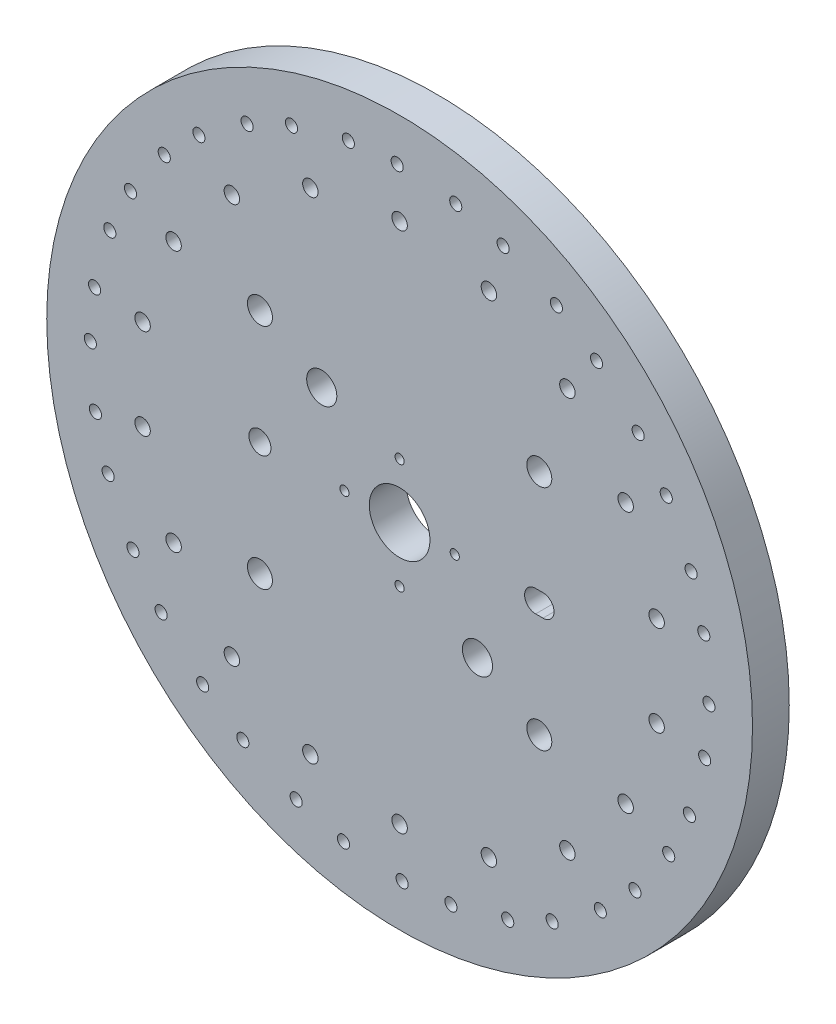
SolidWorks part; units mm, degrees
material "AISI 304"
ref_plane "Front Plane" through (0, 0, 0) normal (0, 0, 1) x (1, 0, 0)
ref_plane "Top Plane" through (0, 0, 0) normal (0, 1, 0) x (1, 0, 0)
ref_plane "Right Plane" through (0, 0, 0) normal (1, 0, 0) x (0, 0, -1)
sketch "Sketch1" plane through (0, 0, 0) normal (0, 0, 1) x (1, 0, 0)
  circle A0 centre (0, 0) radius 102.5
  dimension "D1" = 205
extrude "Boss-Extrude1" add sketch "Sketch1" along normal blind 10
sketch "Sketch2" plane through (0, 0, 0) normal (0, 0, -1) x (-1, 0, 0)
  circle A0 centre (0, 0) radius 8.25
  dimension "D1" = 16.5
extrude "Cut-Extrude1" cut sketch "Sketch2" against normal through all
sketch "Sketch4" plane through (0, 0, 0) normal (0, 0, -1) x (-1, 0, 0)
  line L0 (0, 0) -> (0, -50000) construction
  line L1 (0, 0) -> (-12940.9523, -48296.2913) construction
  circle A0 centre (0, 0) radius 84.145 construction
  circle A1 centre (-29.4071, -78.8391) radius 1
  circle A2 centre (-13.9523, -82.9802) radius 1
  dimension "D1" = 168.29
  dimension "D2" = 16
  dimension "D3" = 2
  dimension "D4" = 15
extrude "Cut-Extrude3" cut sketch "Sketch4" against normal blind 20
pattern_circular "CirPattern2" count 18 over 360 about axis through (0, 0, 0) along (0, 0, 1) of "Cut-Extrude3"
sketch "Sketch5" plane through (0, 0, 0) normal (0, 0, -1) x (-1, 0, 0)
  line L0 (0, 0) -> (0, 50000) construction
  circle A0 centre (0, 0) radius 71 construction
  circle A1 centre (0, -71) radius 2.1
  dimension "D1" = 142
  dimension "D2" = 4.2
extrude "Cut-Extrude4" cut sketch "Sketch5" against normal through all
pattern_circular "CirPattern3" count 18 over 360 about axis through (0, 0, 0) along (0, 0, 1) of "Cut-Extrude4"
sketch "Sketch7" plane through (0, 0, 0) normal (0, 0, -1) x (-1, 0, 0)
  circle A0 centre (0, 0) radius 96
  circle A1 centre (0, 0) radius 102.5
  dimension "D1" = 192
  dimension "D2" = 205
extrude "Cut-Extrude5" cut sketch "Sketch7" against normal blind 34
hole_wizard "M4 Tapped Hole1" positions "3DSketch3" profile "Sketch20" tap size "M4" standard "Gb" end condition through all
sketch3d "3DSketch3"
  line L0 (-15.2701, -82.7478, 10) -> (-15.2701, -82.7478, 0) construction
  line L1 (-28.1497, -79.2968, 10) -> (-28.1497, -79.2968, 0) construction
  line L2 (-42.6506, -72.5349, 10) -> (-42.6506, -72.5349, 0) construction
  line L3 (-53.5731, -64.8868, 10) -> (-53.5731, -64.8868, 0) construction
  line L4 (-64.8868, -53.5731, 10) -> (-64.8868, -53.5731, 0) construction
  line L5 (-72.5349, -42.6506, 10) -> (-72.5349, -42.6506, 0) construction
  line L6 (-79.2968, -28.1497, 10) -> (-79.2968, -28.1497, 0) construction
  line L7 (-82.7478, -15.2701, 10) -> (-82.7478, -15.2701, 0) construction
  line L8 (-84.1423, 0.6691, 10) -> (-84.1423, 0.6691, 0) construction
  line L9 (-82.9802, 13.9523, 10) -> (-82.9802, 13.9523, 0) construction
  line L10 (-78.8391, 29.4071, 10) -> (-78.8391, 29.4071, 0) construction
  line L11 (-73.2039, 41.4917, 10) -> (-73.2039, 41.4917, 0) construction
  line L12 (-64.0267, 54.5982, 10) -> (-64.0267, 54.5982, 0) construction
  line L13 (-54.5982, 64.0267, 10) -> (-54.5982, 64.0267, 0) construction
  line L14 (-41.4917, 73.2039, 10) -> (-41.4917, 73.2039, 0) construction
  line L15 (-29.4071, 78.8391, 10) -> (-29.4071, 78.8391, 0) construction
  line L16 (-13.9523, 82.9802, 10) -> (-13.9523, 82.9802, 0) construction
  line L17 (-0.6691, 84.1423, 10) -> (-0.6691, 84.1423, 0) construction
  line L18 (15.2701, 82.7478, 10) -> (15.2701, 82.7478, 0) construction
  line L19 (28.1497, 79.2968, 10) -> (28.1497, 79.2968, 0) construction
  line L20 (42.6506, 72.5349, 10) -> (42.6506, 72.5349, 0) construction
  line L21 (53.5731, 64.8868, 10) -> (53.5731, 64.8868, 0) construction
  line L22 (64.8868, 53.5731, 10) -> (64.8868, 53.5731, 0) construction
  line L23 (72.5349, 42.6506, 10) -> (72.5349, 42.6506, 0) construction
  line L24 (79.2968, 28.1497, 10) -> (79.2968, 28.1497, 0) construction
  line L25 (82.7478, 15.2701, 10) -> (82.7478, 15.2701, 0) construction
  line L26 (84.1423, -0.6691, 10) -> (84.1423, -0.6691, 0) construction
  line L27 (82.9802, -13.9523, 10) -> (82.9802, -13.9523, 0) construction
  line L28 (78.8391, -29.4071, 10) -> (78.8391, -29.4071, 0) construction
  line L29 (73.2039, -41.4917, 10) -> (73.2039, -41.4917, 0) construction
  line L30 (64.0267, -54.5982, 10) -> (64.0267, -54.5982, 0) construction
  line L31 (54.5982, -64.0267, 10) -> (54.5982, -64.0267, 0) construction
  line L32 (41.4917, -73.2039, 10) -> (41.4917, -73.2039, 0) construction
  line L33 (29.4071, -78.8391, 10) -> (29.4071, -78.8391, 0) construction
  line L34 (13.9523, -82.9802, 10) -> (13.9523, -82.9802, 0) construction
  line L35 (0.6691, -84.1423, 10) -> (0.6691, -84.1423, 0) construction
  point P0 (-15.2701, -82.7478, 10)
  point P5 (-28.1497, -79.2968, 10)
  point P9 (-42.6506, -72.5349, 10)
  point P13 (-53.5731, -64.8868, 10)
  point P17 (-64.8868, -53.5731, 10)
  point P21 (-72.5349, -42.6506, 10)
  point P25 (-79.2968, -28.1497, 10)
  point P29 (-82.7478, -15.2701, 10)
  point P33 (-84.1423, 0.6691, 10)
  point P37 (-82.9802, 13.9523, 10)
  point P41 (-78.8391, 29.4071, 10)
  point P45 (-73.2039, 41.4917, 10)
  point P49 (-64.0267, 54.5982, 10)
  point P53 (-54.5982, 64.0267, 10)
  point P57 (-41.4917, 73.2039, 10)
  point P61 (-29.4071, 78.8391, 10)
  point P65 (-13.9523, 82.9802, 10)
  point P69 (-0.6691, 84.1423, 10)
  point P73 (15.2701, 82.7478, 10)
  point P77 (28.1497, 79.2968, 10)
  point P81 (42.6506, 72.5349, 10)
  point P85 (53.5731, 64.8868, 10)
  point P89 (64.8868, 53.5731, 10)
  point P93 (72.5349, 42.6506, 10)
  point P97 (79.2968, 28.1497, 10)
  point P101 (82.7478, 15.2701, 10)
  point P105 (84.1423, -0.6691, 10)
  point P109 (82.9802, -13.9523, 10)
  point P113 (78.8391, -29.4071, 10)
  point P117 (73.2039, -41.4917, 10)
  point P121 (64.0267, -54.5982, 10)
  point P125 (54.5982, -64.0267, 10)
  point P129 (41.4917, -73.2039, 10)
  point P133 (29.4071, -78.8391, 10)
  point P137 (13.9523, -82.9802, 10)
  point P141 (0.6691, -84.1423, 10)
sketch "Sketch20" plane through (-15.2701, -82.7478, 10) normal (1, 0, 0) x (0, -1, 0)
  line L0 (0, 0) -> (0, 10)
  line L1 (0, 10) -> (1.65, 10)
  line L2 (1.65, 10) -> (1.65, 0)
  line L5 (1.65, 0) -> (0, 0)
  line L11 (0, -6.35) -> (0, 107.95) construction
  dimension "通孔螺纹孔钻头直径" = 3.3
  dimension "通孔螺纹孔钻头深度" = 10
cosmetic thread "Cosmetic thread 17" parameters "D2"=4
cosmetic thread "Cosmetic thread 18" parameters "D2"=4
cosmetic thread "Cosmetic thread 19" parameters "D2"=4
cosmetic thread "Cosmetic thread 20" parameters "D2"=4
cosmetic thread "Cosmetic thread 21" parameters "D2"=4
cosmetic thread "Cosmetic thread 22" parameters "D2"=4
cosmetic thread "Cosmetic thread 23" parameters "D2"=4
cosmetic thread "Cosmetic thread 24" parameters "D2"=4
cosmetic thread "Cosmetic thread 25" parameters "D2"=4
cosmetic thread "Cosmetic thread 26" parameters "D2"=4
cosmetic thread "Cosmetic thread 27" parameters "D2"=4
cosmetic thread "Cosmetic thread 28" parameters "D2"=4
cosmetic thread "Cosmetic thread 29" parameters "D2"=4
cosmetic thread "Cosmetic thread 30" parameters "D2"=4
cosmetic thread "Cosmetic thread 31" parameters "D2"=4
cosmetic thread "Cosmetic thread 32" parameters "D2"=4
cosmetic thread "Cosmetic thread 33" parameters "D2"=4
cosmetic thread "Cosmetic thread 34" parameters "D2"=4
cosmetic thread "Cosmetic thread 35" parameters "D2"=4
cosmetic thread "Cosmetic thread 36" parameters "D2"=4
cosmetic thread "Cosmetic thread 37" parameters "D2"=4
cosmetic thread "Cosmetic thread 38" parameters "D2"=4
cosmetic thread "Cosmetic thread 39" parameters "D2"=4
cosmetic thread "Cosmetic thread 40" parameters "D2"=4
cosmetic thread "Cosmetic thread 41" parameters "D2"=4
cosmetic thread "Cosmetic thread 42" parameters "D2"=4
cosmetic thread "Cosmetic thread 43" parameters "D2"=4
cosmetic thread "Cosmetic thread 44" parameters "D2"=4
cosmetic thread "Cosmetic thread 45" parameters "D2"=4
cosmetic thread "Cosmetic thread 46" parameters "D2"=4
cosmetic thread "Cosmetic thread 47" parameters "D2"=4
cosmetic thread "Cosmetic thread 48" parameters "D2"=4
cosmetic thread "Cosmetic thread 49" parameters "D2"=4
cosmetic thread "Cosmetic thread 50" parameters "D2"=4
cosmetic thread "Cosmetic thread 51" parameters "D2"=4
cosmetic thread "Cosmetic thread 52" parameters "D2"=4
hole_wizard "M8 Tapped Hole2" positions "Sketch40" profile "Sketch39" tap size "M8" standard "Gb" end condition through all
sketch "Sketch40" plane through (0, 0, 10) normal (0, 0, 1) x (1, 0, 0)
  line L0 (0, 0) -> (0, 50000) construction
  line L1 (0, 0) -> (50000, 0) construction
  line L12 (0, 0) -> (35355.3391, 35355.3391) construction
  line L13 (0, 0) -> (38743.251, 31606.3364) construction
  line L14 (0, 0) -> (-38743.251, 31606.3364) construction
  line L15 (0, 0) -> (50000, 0) construction
  circle A0 centre (0, 0) radius 49.0408 construction
  point P0 (-38, 31)
  point P3 (-38, -31)
  point P6 (38, 31)
  point P9 (38, -31)
  dimension "D2" = 98.0816
  dimension "D1" = 45
  dimension "D3" = 0
  dimension "D4" = 101.586
sketch "Sketch39" plane through (-38, 31, 10) normal (1, 0, 0) x (0, -1, 0)
  line L0 (0, 0) -> (0, 10)
  line L1 (0, 10) -> (3.4, 10)
  line L2 (3.4, 10) -> (3.4, 0)
  line L5 (3.4, 0) -> (0, 0)
  line L11 (0, -6.35) -> (0, 107.95) construction
  dimension "通孔螺纹孔钻头直径" = 6.8
  dimension "通孔螺纹孔钻头深度" = 10
cosmetic thread "Cosmetic thread 77" parameters "D2"=8
cosmetic thread "Cosmetic thread 78" parameters "D2"=8
cosmetic thread "Cosmetic thread 79" parameters "D2"=8
cosmetic thread "Cosmetic thread 80" parameters "D2"=8
sketch "Sketch41" plane through (0, 0, 10) normal (0, 0, 1) x (1, 0, 0)
  line L0 (0, 0) -> (0, 50000) construction
  line L1 (0, 0) -> (50000, 0) construction
  circle A0 centre (0, 0) radius 15 construction
  point P3 (0, 15)
  point P8 (15, 0)
  point P9 (0, -15)
  point P10 (-15, 0)
  dimension "D1" = 30
hole_wizard "M3 Tapped Hole1" positions "3DSketch4" profile "Sketch43" tap size "M3" standard "Gb" end condition through all
sketch3d "3DSketch4"
  point P0 (0, 15, 10)
  point P3 (15, 0, 10)
  point P6 (0, -15, 10)
  point P9 (-15, 0, 10)
sketch "Sketch43" plane through (0, 15, 10) normal (1, 0, 0) x (0, -1, 0)
  line L0 (0, 0) -> (0, 10)
  line L1 (0, 10) -> (1.25, 10)
  line L2 (1.25, 10) -> (1.25, 0)
  line L5 (1.25, 0) -> (0, 0)
  line L11 (0, -6.35) -> (0, 107.95) construction
  dimension "通孔螺纹孔钻头直径" = 2.5
  dimension "通孔螺纹孔钻头深度" = 10
cosmetic thread "Cosmetic thread 81" parameters "D1"=10, "D2"=3
cosmetic thread "Cosmetic thread 82" parameters "D1"=10, "D2"=3
cosmetic thread "Cosmetic thread 83" parameters "D1"=10, "D2"=3
cosmetic thread "Cosmetic thread 84" parameters "D1"=10, "D2"=3
sketch "Sketch44" plane through (0, 0, 10) normal (0, 0, 1) x (1, 0, 0)
  line L0 (0, 0) -> (0, 50000) construction
  line L1 (0, 0) -> (-35305.9016, 35404.7075) construction
  circle A0 centre (21.1835, -21.2428) radius 4.1
  circle A1 centre (-21.1835, 21.2428) radius 4.1
  circle A2 centre (0, 0) radius 30 construction
  dimension "D2" = 8.2
  dimension "D3" = 60
  dimension "D1" = 44.92
extrude "Cut-Extrude19" cut sketch "Sketch44" against normal blind 10
sketch "Sketch45" plane through (0, 0, 10) normal (0, 0, 1) x (1, 0, 0)
  line L0 (-38, 0) -> (49962, 0) construction
  circle A0 centre (-38, 0) radius 3
  circle A1 centre (38, 0) radius 3
  circle A2 centre (0, 0) radius 38 construction
  dimension "D1" = 6
  dimension "D2" = 76
extrude "Cut-Extrude20" cut sketch "Sketch45" against normal blind 10
sketch "Sketch47" plane through (0, 0, 10) normal (0, 0, 1) x (1, 0, 0)
  line L0 (37, 0) -> (39, 0) construction
  line L1 (37, 3) -> (39, 3)
  line L2 (37, -3) -> (39, -3)
  arc A0 (37, 3) -> (37, -3) centre (37, 0) ccw
  arc A1 (39, -3) -> (39, 3) centre (39, 0) ccw
  point P2 (38, 0)
  dimension "D1" = 6
  dimension "D2" = 2
extrude "Cut-Extrude21" cut sketch "Sketch47" against normal through all
